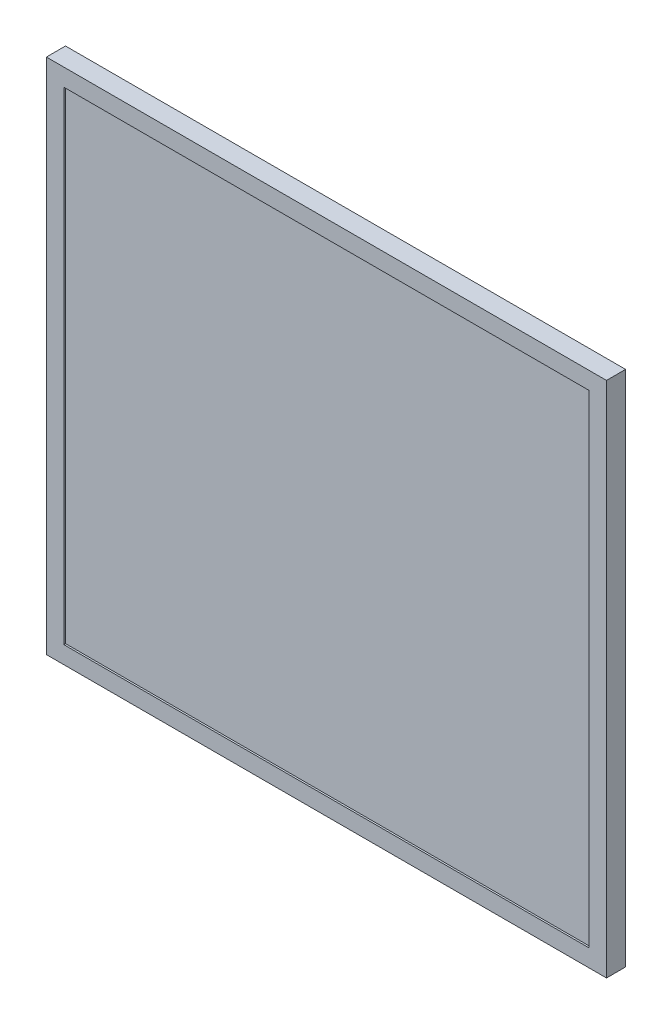
from build123d import *

# Parameters (mm, degrees)
SKETCH_1_W      = 645
SKETCH_1_H      = 596
EXTRUDE_1_DEPTH = 22
SHELL_1_T       = -2
SKETCH_2_W      = 645
SKETCH_2_H      = 596
SKETCH_2_W_2    = 605
SKETCH_2_H_2    = 556
EXTRUDE_2_DEPTH = 2


with BuildPart() as part:
    # 草图1 → 凸台-拉伸1 (new body)
    with BuildSketch(Plane.XY):
        with Locations((322.5, 298)):
            Rectangle(SKETCH_1_W, SKETCH_1_H)
    extrude(amount=EXTRUDE_1_DEPTH)

    # 抽壳1
    shell_1_openings = [part.faces().sort_by_distance(p)[0] for p in [
        (322.5, 298, 22),
    ]]
    offset(amount=SHELL_1_T, openings=shell_1_openings, kind=Kind.INTERSECTION)

    # 草图2 → 凸台-拉伸2 (add)
    with BuildSketch(Plane.XY.offset(22)):
        with Locations((322.5, 298)):
            Rectangle(SKETCH_2_W, SKETCH_2_H)
        with Locations((322.5, 298)):
            Rectangle(SKETCH_2_W_2, SKETCH_2_H_2, mode=Mode.SUBTRACT)
    extrude(amount=-EXTRUDE_2_DEPTH)


solid = part.part
